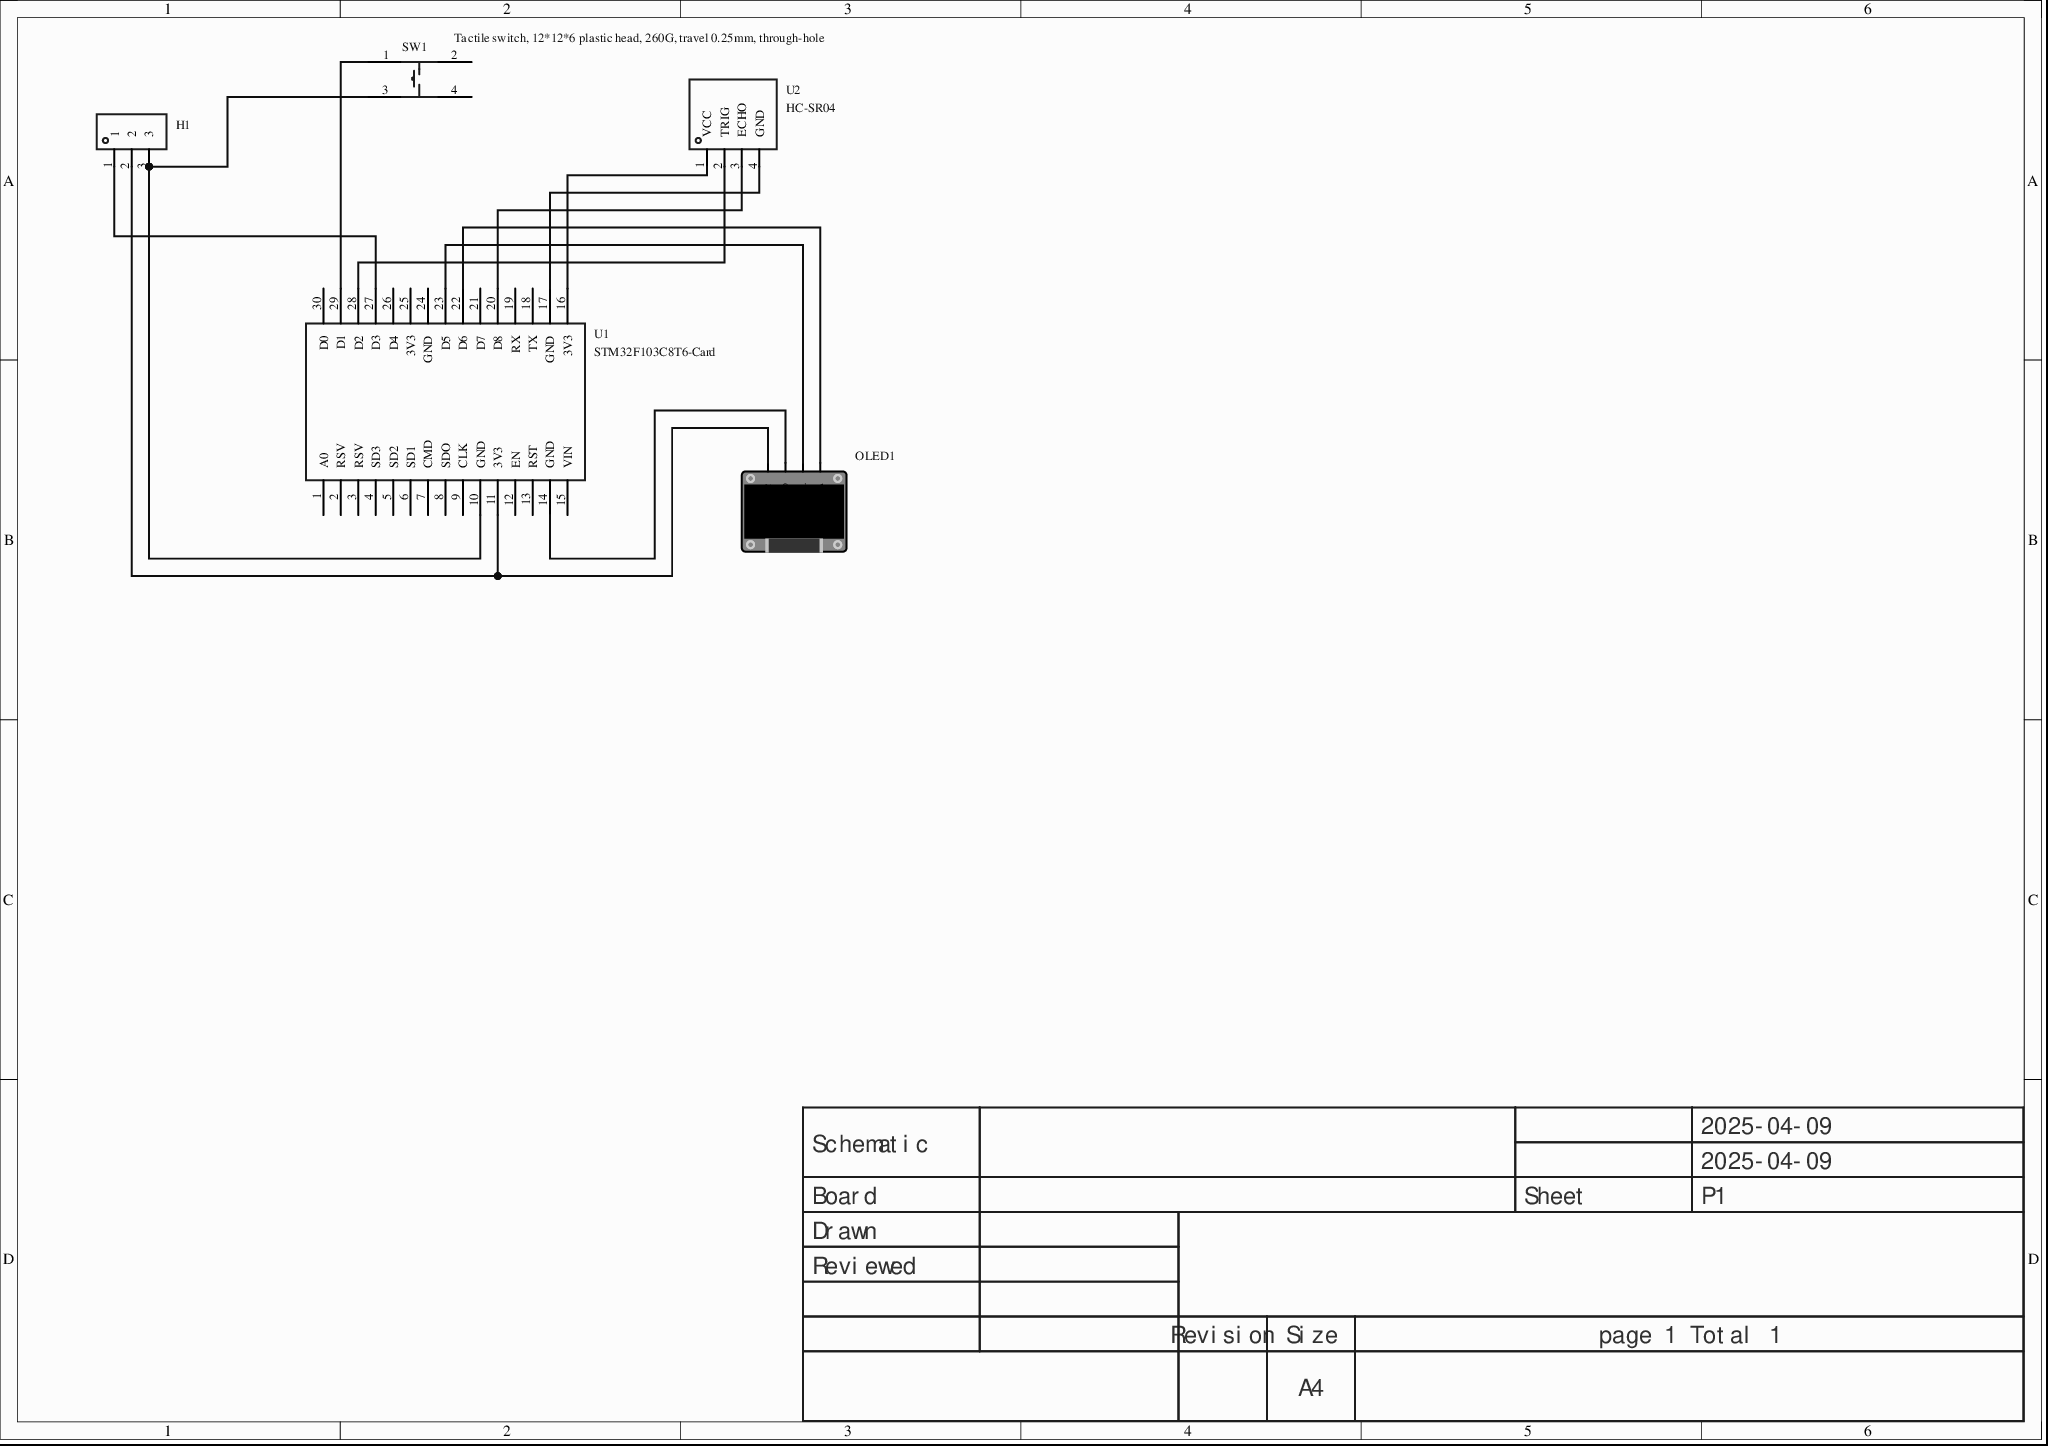
[diagram p0: MISC89069-3.schdoc]
# Altium project MISC89069-2.PrjPcb
1 sheet, 5 parts. Net scope: global (net labels, ports and power ports of the same name join across sheets).
Board file: MISC89069.pcbdoc

## Sheet MISC89069-3.schdoc
size 297 x 209 mm; Version: V1.0; @Project Name: MISC89069; @Page Count: 1; @Update Date: 2025-04-09; @Create Date: 2025-04-09; @Schematic Name: MISC89069; @Page No: 1; @Create Time: 12:54:04; @Update Time: 12:56:05; @Board Name: MISC89069

### Parts
H1  (no value)  [HDR-TH_3P-P2.54-V-F]
OLED1  (no value)  [0.96OLED_4P]
SW1  Tactile switch, 12*12*6 plastic head, 260G, travel 0.25mm, through-hole  [KEY-TH_4P-L12.0-W12.0-P5.00-LS12.5]
U1  STM32F103C8T6-Card  [CONN-TH_L53.3-W22.9_STM32F103C8T6-CARD]
U2  HC-SR04  [TH_HC-SR04V]

### Nets
NetH1_1: H1.1 U1.27(D3)
NetH1_2: H1.2 OLED1.1(VCC) U1.11(3V3)
NetH1_3: H1.3 SW1.3 U1.10(GND)
NetOLED1_2: OLED1.2(GND) U1.14(GND)
NetOLED1_3: OLED1.3(SCL) U1.23(D5)
NetOLED1_4: OLED1.4(SDA) U1.22(D6)
NetSW1_1: SW1.1 U1.29(D1)
NetU1_16: U1.16(3V3) U2.1(VCC)
NetU1_17: U1.17(GND) U2.4(GND)
NetU1_20: U1.20(D8) U2.3(ECHO)
NetU1_28: U1.28(D2) U2.2(TRIG)

Not connected (* = marked no-connect by the designer): SW1 2 4; U1 1(A0) 2(RSV) 3(RSV) 4(SD3) 5(SD2) 6(SD1) 7(CMD) 8(SDO) 9(CLK) 12(EN) 13(RST) 15(VIN) 18(TX) 19(RX) 21(D7) 24(GND) 25(3V3) 26(D4) 30(D0)

### Notes on the sheet
- 2025-04-09
- Schematic
- Board
- Sheet
- P1
- Drawn
- Reviewed
- Revision
- Size
- A4
- page 1 Total 1

### Library data of the parts
H1 = HDR-F_2.54_1x3P: Symbol: PM254V-11-03-H85; ConvertToPcb: yes; ModelId: f3b3cc5aae9641bf9e56fc160cef875b; ModelName: HDR2.54-F-LI-1X3P; ModelTransform: 299.9994,100,0,0,0,0,0,0,-118.11; Device: HDR-F_2.54_1x3P; AddInBom: yes; SupplierPart: C541850; Supplier Footprint: 插件; FootprintName: HDR-TH_3P-P2.54-V-F
OLED1 = 0.96OLED模块_4P: Device: 0.96OLED module_4P; ConvertToPcb: yes; ModelId: 79c000fdb68d45a296c2e9bedf4f9055; ModelTransform: 1393.69792,1318.895,0,0,0,0,0,-560.079,-137.795; AddInBom: yes; Supplier Footprint: 插件; SymbolName: 0.96OLED module_4P; FootprintName: 0.96OLED_4P; ModelName: 0.96OLED_4P
SW1 = 轻触开关,12*12*6塑头,260G,行程0.25mm,直插: Symbol: SWITCH,12*12*6PLASTIC HEAD,260G, 0.25MM,STRAIGHT LINE; AddInBom: yes; ModelId: 58bd23e2e6df4c6ea4917606aab27058; ModelTransform: 542.968,472.44,0,0,0,0,0,0,-137.795; Device: Tactile switch, 12*12*6 plastic head, 260G, travel 0.25mm, through-hole; LCSC Part Name: 轻触开关,12*12*6塑头,260G,行程0.25mm,直插; SupplierPart: C71860; ManufacturerPart: 轻触开关,12*12*6塑头,260G,行程0.25mm,直插; Supplier Footprint: 插件; JLCPCB Part Class: Extended library; Supplier: LCSC; ConvertToPcb: yes; FootprintName: KEY-TH_4P-L12.0-W12.0-P5.00-LS12.5; ModelName: KEY-TH_4P-L12.0-W12.0-P5.00-LS12.5
U1 = STM32F103C8T6-Card: AddInBom: yes; Symbol: STM32F103C8T6-CARD; Device: STM32F103C8T6-Card; LCSC Part Name: STM32F103C8T6-Card; SupplierPart: C9900077949; ManufacturerPart: STM32F103C8T6-Card; Supplier Footprint: 插件; Supplier: LCSC; ConvertToPcb: yes; FootprintName: CONN-TH_L53.3-W22.9_STM32F103C8T6-CARD
U2 = HC-SR04: Manufacturer: Universal Microelectronics; AddInBom: yes; Symbol: HC-SR04; Device: HC-SR04; LCSC Part Name: HC-SR04; SupplierPart: C19857336; ManufacturerPart: HC-SR04; Supplier Footprint: -; JLCPCB Part Class: Extended library; Datasheet: example.com/20240122/47B8E374E428935B7962A2189EF91AAC.pdf; Supplier: LCSC; ConvertToPcb: yes; FootprintName: TH_HC-SR04V